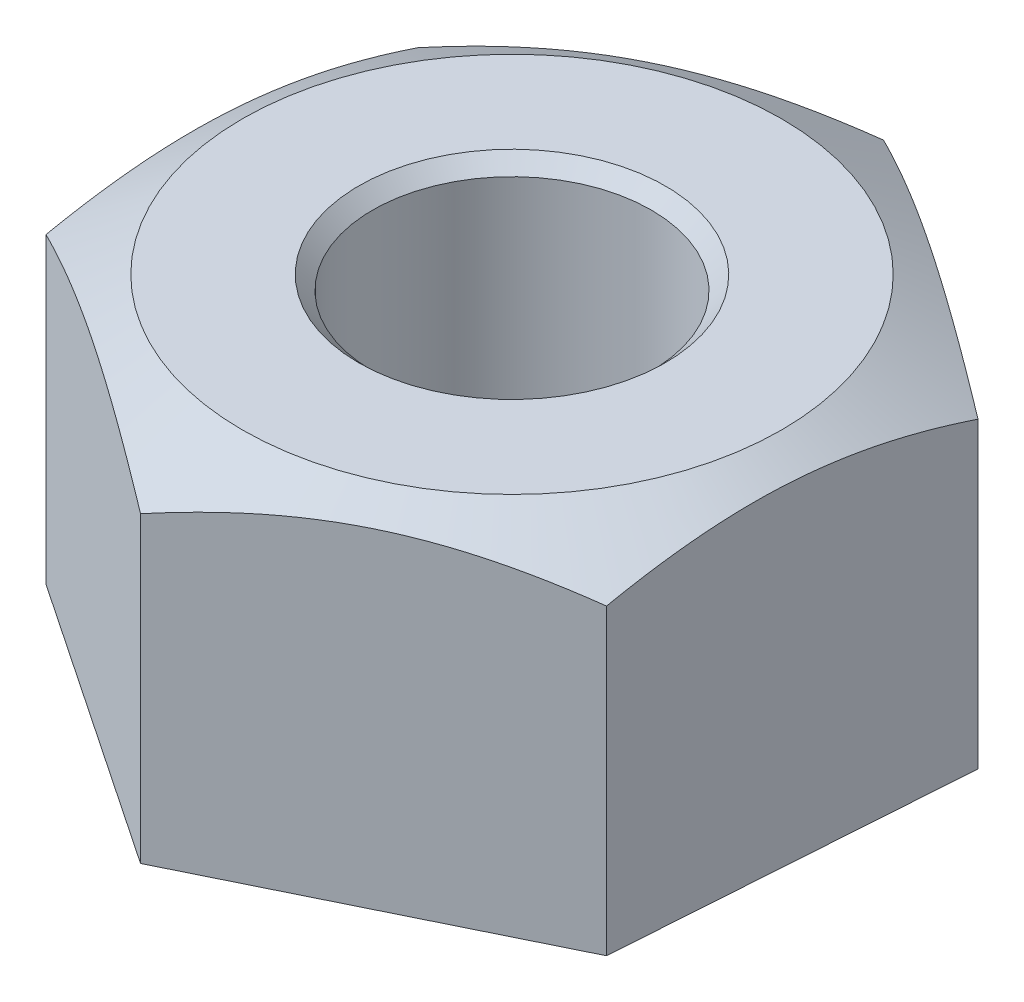
from build123d import *

# Parameters (mm, degrees)
SKETCH1_R           = 2
BOSS_EXTRUDE1_DEPTH = 5
SKETCH8_OUTSIDE_W   = 31.17
SKETCH8_OUTSIDE_H   = 32.162
SKETCH8_OUTSIDE_R   = 3.869068986
CUT_EXTRUDE1_DEPTH  = 5
CUT_EXTRUDE1_DRAFT  = -60
CHAMFER1_SIZE       = 0.2
CHAMFER2_SIZE       = 0.2


with BuildPart() as part:
    # Sketch1 → Boss-Extrude1 (new body)
    with BuildSketch(Plane(origin=(0, 0, 0), x_dir=(1, 0, 0), z_dir=(0, 1, 0))):
        Polygon((4.148216558, -2.791469037), (4.491591379, 2.196726401), (0.343374821, 4.988195438), (-4.148216558, 2.791469037), (-4.491591379, -2.196726401), (-0.343374821, -4.988195438), align=None)
        with Locations(Location((0, 0, 0), (0, 0, 270))):
            Circle(SKETCH1_R, mode=Mode.SUBTRACT)
    extrude(amount=BOSS_EXTRUDE1_DEPTH)


with BuildPart() as cut_extrude1_tool:
    # Sketch8 outside → Cut-Extrude1 (with draft: the straight prism first)
    with BuildSketch(Plane(origin=(0, 5, 0), x_dir=(1, 0, 0), z_dir=(0, 1, 0))):
        Rectangle(SKETCH8_OUTSIDE_W, SKETCH8_OUTSIDE_H)
        Circle(SKETCH8_OUTSIDE_R, mode=Mode.SUBTRACT)
    extrude(amount=-CUT_EXTRUDE1_DEPTH)
    # Cut-Extrude1: the draft: its side faces are tilted about the plane it starts from
    cut_extrude1_sides = [cut_extrude1_tool.faces().sort_by_distance(p)[0] for p in [
        (0, 2.5, 16.081),
        (15.585, 2.5, 0),
        (0, 2.5, -16.081),
        (-15.585, 2.5, 0),
        (-3.869068986, 2.5, 0),
    ]]
    draft(cut_extrude1_sides, Plane(origin=(0, 5, 0), x_dir=(1, 0, 0), z_dir=(0, 1, 0)), CUT_EXTRUDE1_DRAFT)


with BuildPart() as part_1:
    add(part.part)

    # Cut-Extrude1: cut by cut_extrude1_tool
    add(cut_extrude1_tool.part, mode=Mode.SUBTRACT)

    # Chamfer1
    chamfer1_edges = [part_1.edges().sort_by_distance(p)[0] for p in [
        (0, 5, -2),
    ]]
    chamfer(chamfer1_edges, length=CHAMFER1_SIZE)

    # Chamfer2
    chamfer2_edges = [part_1.edges().sort_by_distance(p)[0] for p in [
        (0, 0, -2),
    ]]
    chamfer(chamfer2_edges, length=CHAMFER2_SIZE)


solid = part_1.part
